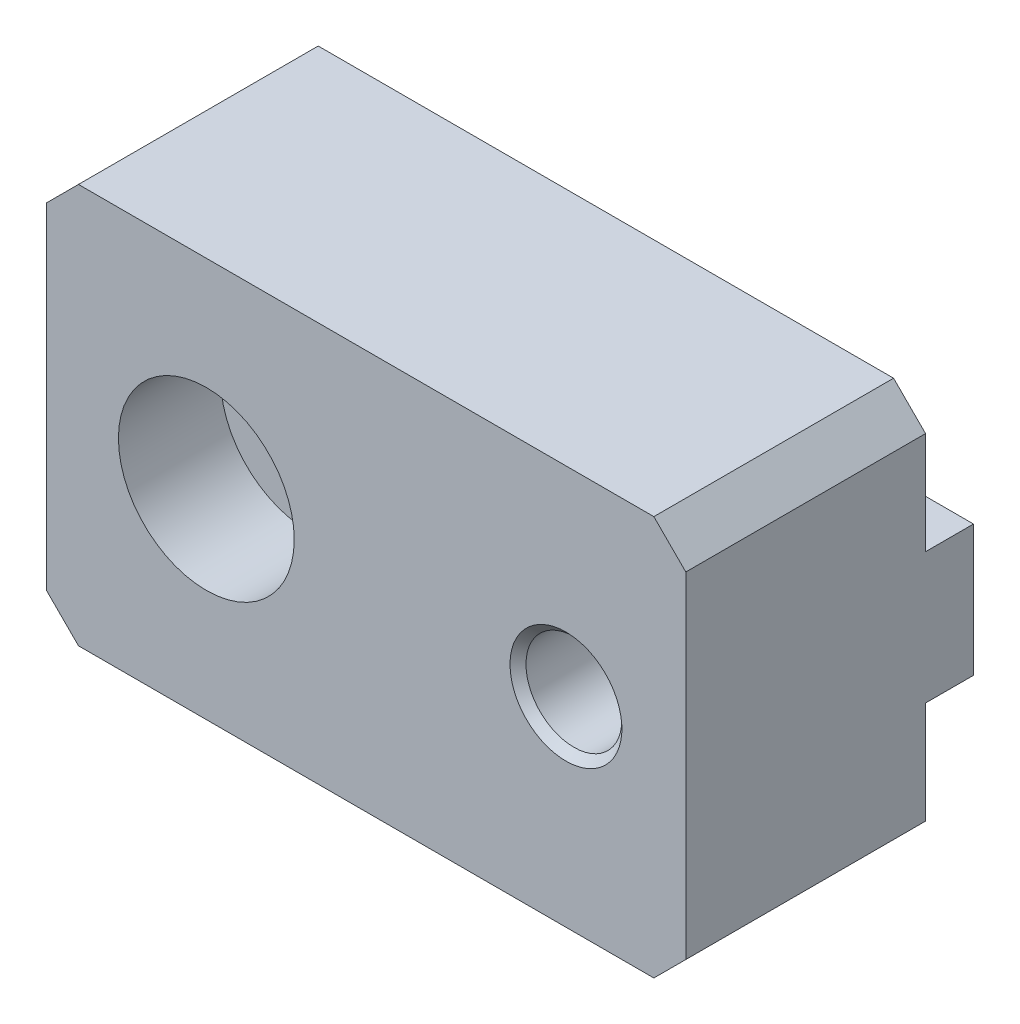
from build123d import *

# Parameters (mm, degrees)
SKETCH_1_W                   = 40
SKETCH_1_H                   = 25
EXTRUDE_1_DEPTH              = 15
SKETCH_9_W                   = 40
SKETCH_9_H                   = 8.2
EXTRUDE_3_DEPTH              = 3
HOLE_WIZARD_M6_2_D           = 6.6
HOLE_WIZARD_M6_2_CBORE_D     = 11
HOLE_WIZARD_M6_2_CBORE_DEPTH = 6.4
SKETCH_12_R                  = 3
CUT_EXTRUDE_3_DEPTH          = 51.487622245
CHAMFER_2_SIZE               = 0.5
CHAMFER_3_SIZE               = 2


with BuildPart() as part:
    # 草图1 → 凸台-拉伸1 (new body)
    with BuildSketch(Plane.XY):
        with Locations((20, 12.5)):
            Rectangle(SKETCH_1_W, SKETCH_1_H)
    extrude(amount=EXTRUDE_1_DEPTH)

    # 草图9 → 凸台-拉伸3 (add)
    with BuildSketch(Plane(origin=(0, 0, 0), x_dir=(-1, 0, 0), z_dir=(0, 0, -1))):
        with Locations((-20, 12.5)):
            Rectangle(SKETCH_9_W, SKETCH_9_H)
    extrude(amount=EXTRUDE_3_DEPTH)

    # M6 六角凹头螺钉的柱形沉头孔2 (through all)
    with Locations(Plane.XY.offset(15)):
        with Locations((10, 12.5)):
            CounterBoreHole(HOLE_WIZARD_M6_2_D / 2, HOLE_WIZARD_M6_2_CBORE_D / 2, HOLE_WIZARD_M6_2_CBORE_DEPTH)

    # 草图12 → 切除-拉伸3 (cut, through all)
    with BuildSketch(Plane.XY.offset(15)):
        with Locations((32.5, 12.5)):
            Circle(SKETCH_12_R)
    extrude(amount=-CUT_EXTRUDE_3_DEPTH, mode=Mode.SUBTRACT)

    # 倒角2
    chamfer_2_edges = [part.edges().sort_by_distance(p)[0] for p in [
        (29.5, 12.5, 15),
    ]]
    chamfer(chamfer_2_edges, length=CHAMFER_2_SIZE)

    # 倒角3
    chamfer_3_edges = [part.edges().sort_by_distance(p)[0] for p in [
        (40, 0, 7.5),
        (0, 0, 7.5),
        (0, 25, 7.5),
        (40, 25, 7.5),
    ]]
    chamfer(chamfer_3_edges, length=CHAMFER_3_SIZE)


solid = part.part
